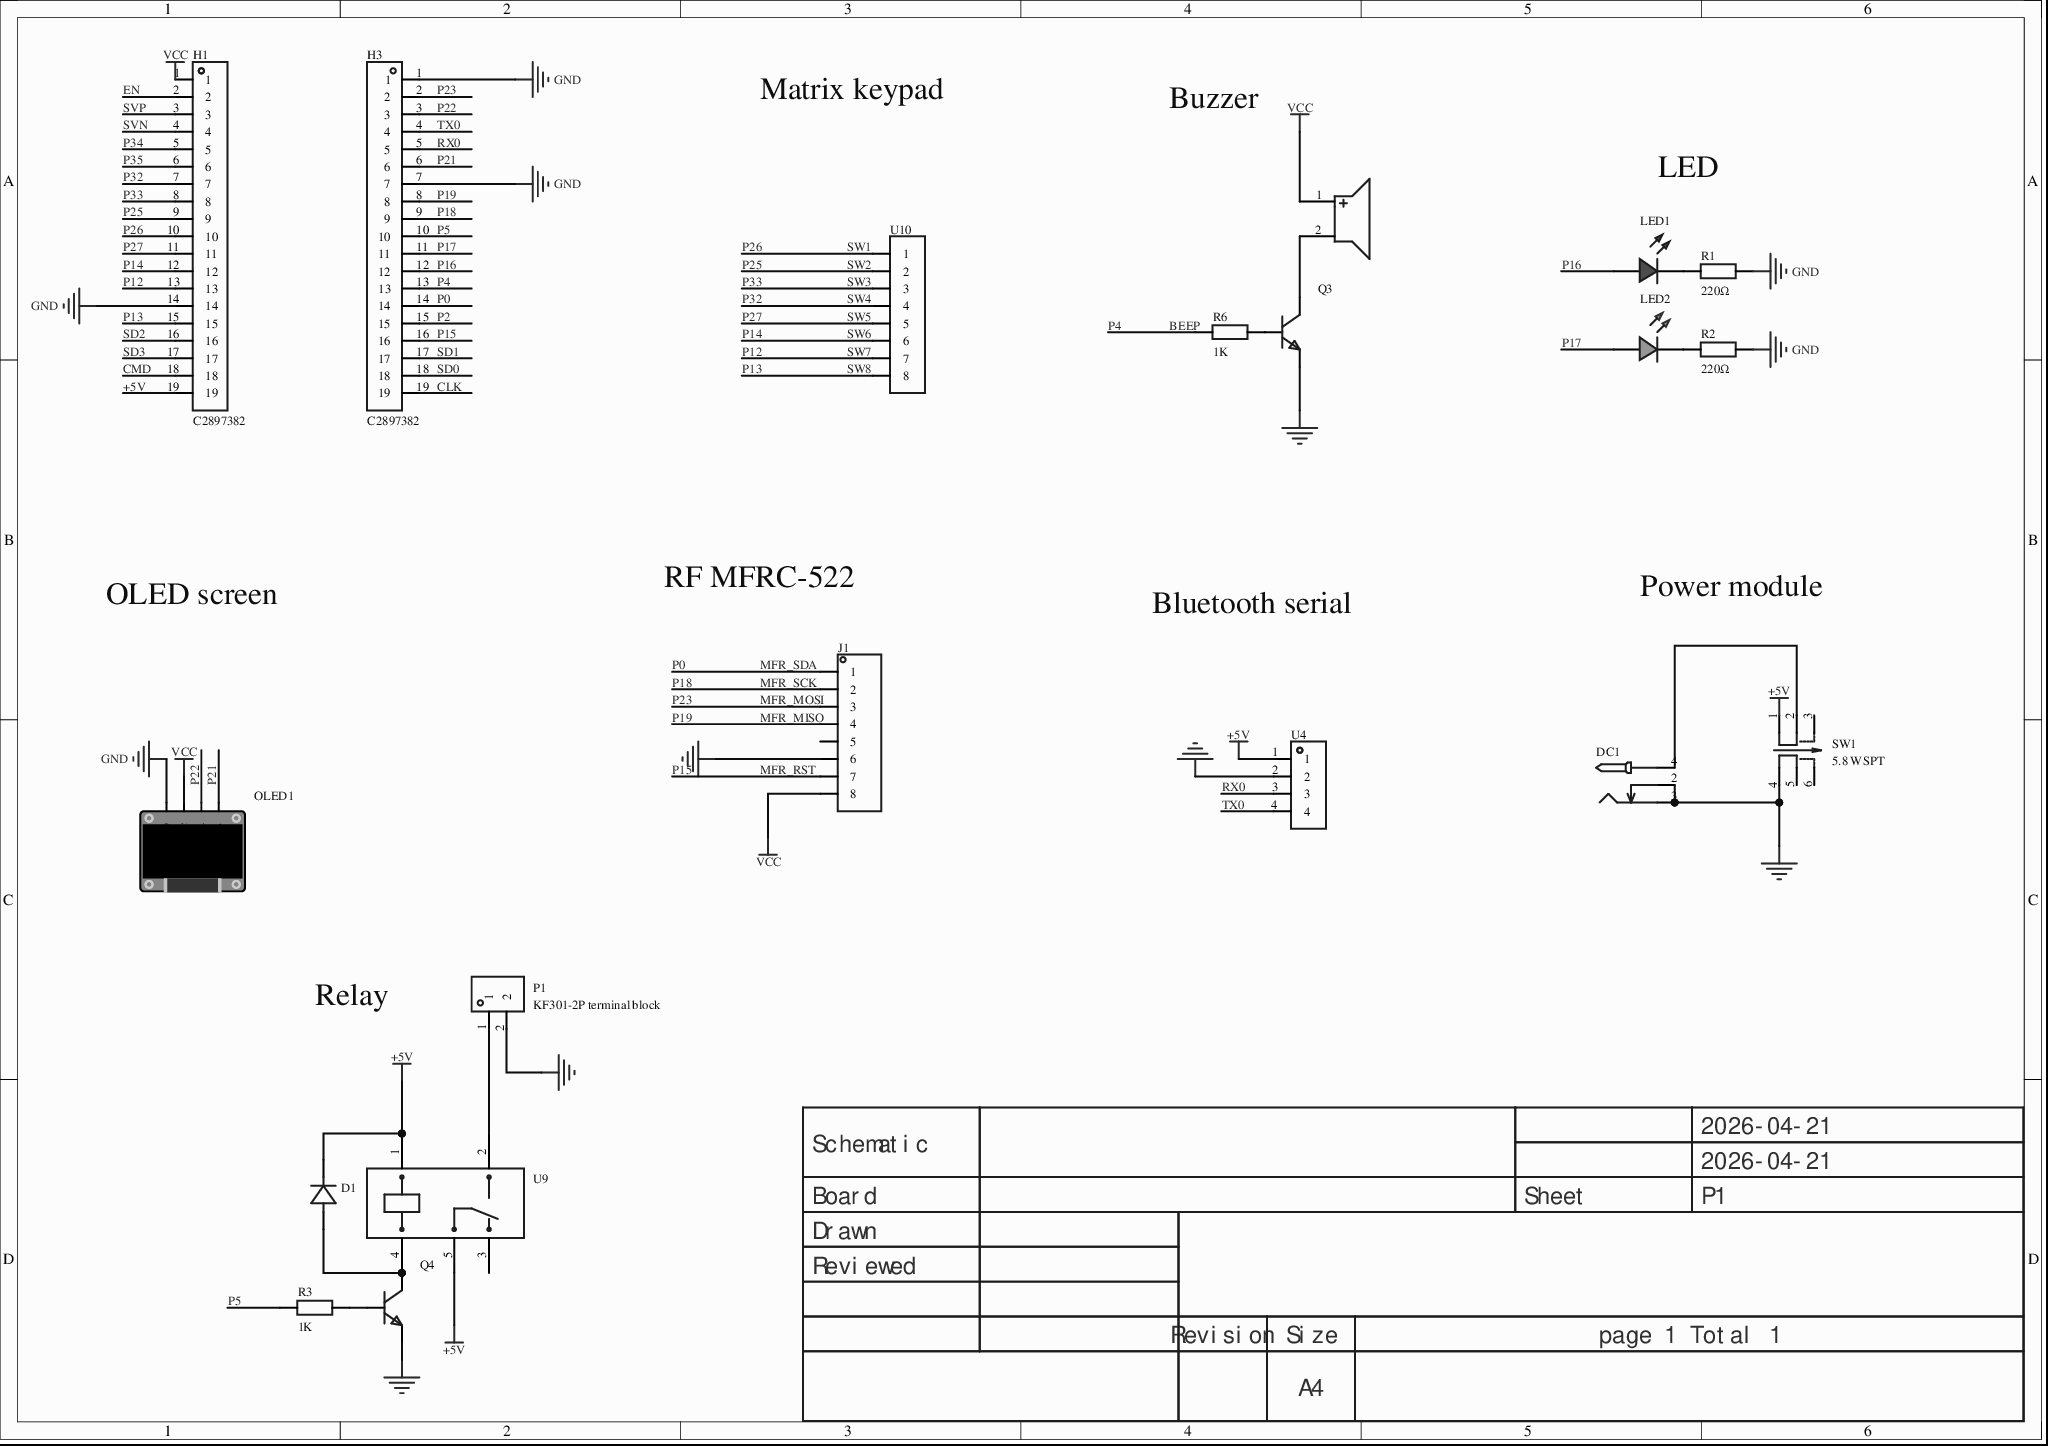
[diagram p0: MISC89084-3.schdoc]
# Altium project MISC89084-2.PrjPcb
1 sheet, 20 parts. Net scope: global (net labels, ports and power ports of the same name join across sheets).
Board file: MISC89084.pcbdoc

## Sheet MISC89084-3.schdoc
size 297 x 209 mm; Version: V1.0; @Project Name: MISC89084; @Page Count: 1; @Update Date: 2026-04-21; @Create Date: 2026-04-21; @Schematic Name: MISC89084; @Page No: 1; @Create Time: 19:02:24; @Update Time: 19:02:29; @Board Name: MISC89084

### Parts
BUZZER1  2.7kHz  [BUZ-TH_BD9.0-P4.00-D0.6-FD]  (value not drawn)
D1  (no value)  [DO_1N4007]
DC1  (no value)  [DC-2.0]
H1  C2897382  [HDR-TH_19P-P2.54-V-F]
H3  C2897382  [HDR-TH_19P-P2.54-V-F]
J1  (no value)  [HDR-TH_8P-P2.54-V-M]
LED1  (no value)  [LED_TH-3mm]
LED2  (no value)  [LED_TH-3mm]
OLED1  (no value)  [0.96OLED_4P]
P1  KF301-2P terminal block  [CONN-TH_XY301V-A-5.0-2P]
Q3  (no value)  [S8050_TO_92]
Q4  (no value)  [S8050_TO_92]
R1  220Ω  [Res_1/8W]
R2  220Ω  [Res_1/8W]
R3  1K  [Res_1/8W]
R6  1K  [Res_1/8W]
SW1  5.8 WSPT  [SW-TH_6P-L5.8-W5.8-P2.00-LS4.5-TL_K8-5851E-L1]
U4  (no value)  [HDR-TH_4P-P2.54-V-F]
U9  SRD-12VDC-SL-C  [RELAY-TH_SRD-XXVDC-XL-C]  (value not drawn)
U10  (no value)  [HDR-TH_8P-P2.54-V-F-1]

### Nets
+5V: D1.1(K) H1.19 SW1.1 U4.1 U9.1 U9.5
GND: DC1.2 DC1.3 H1.14 H3.1 H3.7 J1.6 OLED1.1(GND) P1.2 Q3.1(E) Q4.1(E) R1.2 R2.2 SW1.4 U4.2
VCC: BUZZER1.1 H1.1 J1.8 OLED1.2(VCC)
BEEP: H3.13 R6.1  [also labelled P4]
CLK: H3.19
CMD: H1.18
EN: H1.2
MFR_MISO: H3.8 J1.4  [also labelled P19]
MFR_MOSI: H3.2 J1.3  [also labelled P23]
MFR_RST: H3.16 J1.7  [also labelled P15]
MFR_SCK: H3.9 J1.2  [also labelled P18]
MFR_SDA: H3.14 J1.1  [also labelled P0]
P2: H3.15
P5: H3.10 R3.1
P12: H1.13 U10.7  [also labelled SW7]
P13: H1.15 U10.8  [also labelled SW8]
P14: H1.12 U10.6  [also labelled SW6]
P16: H3.12 LED1.1(C)
P17: H3.11 LED2.1(C)
P21: H3.6 OLED1.4(SDA)
P22: H3.3 OLED1.3(SCL)
P25: H1.9 U10.2  [also labelled SW2]
P26: H1.10 U10.1  [also labelled SW1]
P27: H1.11 U10.5  [also labelled SW5]
P32: H1.7 U10.4  [also labelled SW4]
P33: H1.8 U10.3  [also labelled SW3]
P34: H1.5
P35: H1.6
RX0: H3.5 U4.3
SD0: H3.18
SD1: H3.17
SD2: H1.16
SD3: H1.17
SVN: H1.4
SVP: H1.3
TX0: H3.4 U4.4
NetBUZZER1_2: BUZZER1.2 Q3.3(C)
NetD1_2: D1.2(A) Q4.3(C) U9.4
NetDC1_4: DC1.4 SW1.2
NetLED1_2: LED1.2(A) R1.1
NetLED2_2: LED2.2(A) R2.1
NetP1_1: P1.1 U9.2
NetQ3_2: Q3.2(B) R6.2
NetQ4_2: Q4.2(B) R3.2

Not connected (* = marked no-connect by the designer): J1 5; SW1 3 5 6; U9 3

### Notes on the sheet
- Matrix keypad
- Buzzer
- LED
- OLED screen
- RF MFRC-522
- Power module
- Bluetooth serial
- Relay
- 2026-04-21
- Schematic
- Board
- Sheet
- P1
- Drawn
- Reviewed
- Revision
- Size
- A4
- page 1 Total 1

### Library data of the parts
BUZZER1 = QMB-09B-03: Drive mode: passive (external drive); type: electromagnetic; frequency: 2.7kHz; SPL: 85dB;; Manufacturer: 华能; AddInBom: yes; ModelId: 949096c5110a440bbcfd89e7e6948986; ModelName: BUZ-TH_D9.0-H5.5-P4.0; ModelTransform: 354.33,354.33,0,90,0,0,0,0,-177.165; Voltage - Supply: 2V~5V; Symbol: QMB-09B-03; Device: QMB-09B-03; LCSC Part Name: 无源蜂鸣器QMB-09B-03; SupplierPart: C96256; ManufacturerPart: QMB-09B-03; Supplier Footprint: 插件,D=9mm; JLCPCB Part Class: Extended library; Datasheet: https://atta.szlcsc.com/upload/public/pdf/source/20210401/C96256_958B17753B5AD7CBFBCFFC7C095B4484.pdf; Supplier: LCSC; ConvertToPcb: yes; FootprintName: BUZ-TH_BD9.0-P4.00-D0.6-FD; Driver Circuitry: Passive (external drive); Technology: Electromagnetic; Value: 2.7kHz; Sound Pressure Level(SPL): 85dB; Diameter(φD): 9mm; Height: 5.7mm
D1 = D_1N4007A: AddInBom: yes; ModelId: 6de1e9b71a0d4751b4e9df530304c1a3; ModelName: DO-41_D2.4-L4.7-P8.70; ModelTransform: 373.9,94.4,232.29,0,0,0,0,0,-140; Symbol: D_1N4007; Device: D_1N4007A; Supplier Footprint: DO-41; ConvertToPcb: yes; FootprintName: DO_1N4007
DC1 = DC-005_2.0: Symbol: DC power jack; ConvertToPcb: yes; ModelId: f5f20b8a2308479b936ba3c2698865bb0819f05c4eef4c71ace90d822a990e87; ModelName: DC-IN-TH_DC-5520-1; ModelTransform: 372.05,551.18,582.68,90,0,0,137.8,0,-149.61; Device: DC-005_2.0; AddInBom: yes; Supplier Footprint: 插件; FootprintName: DC-2.0
H1 H3 = HDR-F_2.54_1x19P: ConvertToPcb: yes; ModelId: 131ee080550a465daf9368d356f53fe90819f05c4eef4c71ace90d822a990e87; ModelName: HDR-TH_19P-P2.54-F-LI-1X19P; ModelTransform: 1919.68128,95.6691,0,0,0,0,0,0,-125.984; Symbol: HDR-F_2.54_1x19P; Device: HDR-F_2.54_1x19P; AddInBom: yes; Supplier Footprint: 插件; ManufacturerPart: C2897382; FootprintName: HDR-TH_19P-P2.54-V-F
J1 = HDR-M_2.54_1x8P: Symbol: Header-Male-2.54_1x8; ConvertToPcb: yes; ModelId: f5b96e27511e49e38545e53df2320202; ModelTransform: 807.87244,98.425,0,0,0,0,0,0,-118.11; Device: HDR-M_2.54_1x8P; AddInBom: yes; SupplierPart: C124381; Supplier Footprint: 插件; FootprintName: HDR-TH_8P-P2.54-V-M; ModelName: HDR-TH_8P-P2.54-V-M
LED1 = LED_TH-R_3mm: ConvertToPcb: yes; ModelId: a497c992633541038a38947cdc58012f0819f05c4eef4c71ace90d822a990e87; ModelName: LED-TH-3mm_R; ModelTransform: 141.274,153.327,0,0,0,0,-5.984,0,-137.795; Symbol: LED_TH-R; Device: LED_TH-R_3mm; AddInBom: yes; FootprintName: LED_TH-3mm; Supplier Footprint: 插件
LED2 = LED_TH-G_3mm: AddInBom: yes; ModelId: 07c881668c9448ef9b36eb6a2126ca130819f05c4eef4c71ace90d822a990e87; ModelName: LED-TH-3mm_G; ModelTransform: 141.27444,153.32669525336098,354.32999763315956,0,0,0,-5.90551,0,-137.79528; Symbol: LED_TH-G; Device: LED_TH-G_3mm; ConvertToPcb: yes; FootprintName: LED_TH-3mm; Supplier Footprint: 插件
OLED1 = 0.96OLED模块_4P: Symbol: 0.96OLED module_4P; ConvertToPcb: yes; ModelId: 79c000fdb68d45a296c2e9bedf4f90550819f05c4eef4c71ace90d822a990e87; ModelTransform: 1393.69792,1318.895,0,0,0,0,0,-560.079,-137.795; Device: 0.96OLED module_4P; AddInBom: yes; FootprintName: 0.96OLED_4P; Supplier Footprint: 插件; ModelName: 0.96OLED_4P
P1 = KF301-2P接线端子: AddInBom: yes; ModelId: ef7ead88b0f2448d904975b26718870f0819f05c4eef4c71ace90d822a990e87; ModelTransform: 417.322,299.212,0,0,0,0,11.811,-7.835,-157.48; Symbol: KF301-2P terminal block; Device: KF301-2P terminal block; LCSC Part Name: KF301-2P接线端子; SupplierPart: C9900016950; ManufacturerPart: KF301-2P接线端子; Supplier Footprint: CK301-2P; JLCPCB Part Class: Extended Part; Supplier: LCSC; ConvertToPcb: yes; FootprintName: CONN-TH_XY301V-A-5.0-2P; ModelName: CONN-TH_XY301V-A-5.0-2P
Q3 Q4 = S8050_TO_NPN: ConvertToPcb: yes; ModelId: aafe8e06f2154e7c93506efd0d6632dd; ModelName: TO-92-3_L4.9-W3.7-P1.27-L; ModelTransform: 180.78,141.44,417.3,0,0,0,0,0,-200; Device: S8050_TO_NPN; Symbol: S8050_TO_NPN; AddInBom: yes; Supplier Footprint: TO-92; FootprintName: S8050_TO_92
R1 R2 = Res_AXIAL-1/8W: Symbol: Resistor; 3D Model: b2b5ae7ae4c642178fe0039925c86a3f; 3D Model Transform: 282.86,66.88,253.09,0,0,0,0,0,-191; ConvertToPcb: yes; ModelName: RES-TH_BD1.8-L3.2-P7.20-D0.4; Device: Res_AXIAL-1/8W; Supplier Footprint: 轴向引线; Value: 220Ω; AddInBom: yes; FootprintName: Res_1/8W
R3 = Res_AXIAL-1/8W: Symbol: Resistor; ConvertToPcb: yes; Value: 10kΩ; ModelId: b2b5ae7ae4c642178fe0039925c86a3f; ModelName: RES-TH_BD1.8-L3.2-P7.20-D0.4; ModelTransform: 282.86,66.88,253.09,0,0,0,0,0,-191; Device: Res_AXIAL-1/8W; AddInBom: yes; Supplier Footprint: 轴向引线; FootprintName: Res_1/8W
R6 = Res_AXIAL-1/8W: Symbol: Resistor; ConvertToPcb: yes; ModelId: b2b5ae7ae4c642178fe0039925c86a3f; ModelName: RES-TH_BD1.8-L3.2-P7.20-D0.4; ModelTransform: 282.86,66.88,253.09,0,0,0,0,0,-191; Value: 1K; Device: Res_AXIAL-1/8W; AddInBom: yes; Supplier Footprint: 轴向引线; FootprintName: Res_1/8W
SW1 = 5.8 WSPT: Circuit: DPDT; self-lock/no-lock: no-lock; mounting: through-hole; contact current: 100mA; rated voltage (AC): -; rated voltage (DC): 30V; with lamp: no; actuating force: 1.8N; mechanical life: 5 thousand cycles;; Manufacturer: SHOU HAN(首韩); AddInBom: yes; ModelId: b8faad98a5c645e9866333cdaba903c3; ModelTransform: 229.1334,228.346,0,0,0,0,0,0,-137.795; Actuator Style: Rectangular plunger; Insulation Resistance: 100MΩ; Actuator/Cap Color: Blue; Pin Style: PC pin; Symbol: 5.8 WSPT; Device: 5.8 WSPT; LCSC Part Name: 按键开关5.8x5.8 无锁平头 180gf; SupplierPart: C5379898; ManufacturerPart: 5.8 WSPT; Supplier Footprint: 插件; JLCPCB Part Class: Extended library; Datasheet: https://atta.szlcsc.com/upload/public/pdf/source/20230323/C831DDA43A625CDC196CB35781CDAE7F.pdf; Supplier: LCSC; ConvertToPcb: yes; FootprintName: SW-TH_6P-L5.8-W5.8-P2.00-LS4.5-TL_K8-5851E-L1; ModelName: SW-TH_6P-L5.8-W5.8-P2.00-LS4.5-TL_K8-5851E-L1; Self Lock / No Lock: No-lock; IP Rating: -; Mounting Style: Through-hole; Contact Current: 100mA; Voltage Rating (AC): -; Voltage Rating (DC): 30V; With Lamp: No; Operating Force: 1.8N; Operating Temperature: -10℃~+70℃; Mechanical Life: 5 thousand cycles
U4 = HDR-F_2.54_1x4P: Symbol: 2.54-1*4P female; ConvertToPcb: yes; ModelId: d187812051054f85879fcaa51a310d8e; ModelTransform: 419.6842,98.464,0,0,0,0,0,0,-118.11; Device: HDR-F_2.54_1x4P; AddInBom: yes; SupplierPart: C2718488; Supplier Footprint: 插件; FootprintName: HDR-TH_4P-P2.54-V-F; ModelName: HDR-TH_4P-P2.54-V-F
U9 = SRD-12VDC-SL-C: Coil voltage: 12V; contact form: 1C (SPDT changeover); contact rating (resistive): -; max switching voltage: 250V@AC; max switching current: 15A;; Manufacturer: 松乐; AddInBom: yes; ModelId: d0eda9b8bf8746d18ae810ab88dc78e7; ModelName: RELAY-TH_L19.2-W15.6-H15.8; ModelTransform: 755.904,622.4397,0,0,0,0,34.882,0,-118.11; Pin Number: 5; Coil Rated Power: 360mW; Coil Type: Non-polar, single coil; Coil Resistance: 400Ω; Contact Resistance: 100mΩ; Operate Time: 10ms; Symbol: SRD-12VDC-SL-C; Device: SRD-12VDC-SL-C; LCSC Part Name: SRD-12VDC-SL-C; SupplierPart: C30431; ManufacturerPart: SRD-12VDC-SL-C; Supplier Footprint: 插件,15.6x19.2mm; JLCPCB Part Class: Extended library; Datasheet: https://atta.szlcsc.com/upload/public/pdf/source/20200305/C490149_C96E4098A3B1FFB377D5AD2E40B7C2A8.pdf; Supplier: LCSC; ConvertToPcb: yes; FootprintName: RELAY-TH_SRD-XXVDC-XL-C; Coil Voltage: 12V; Contact Form: 1C (SPDT changeover); Contact Rating: -; Maximum Switching Voltage: 250V@AC; Maximum Switching Current: 15A; Release Time: 10ms
U10 = HDR-F_2.54_1x8P: Symbol: Header-Female-2.54_1x8; AddInBom: yes; ModelId: 0f7e4d9227ef4fa08d5469c22cc70cdb; ModelName: HDR-F-2.54_1x8; ModelTransform: 799.99844,100,0,0,0,0,0,0,-118.11; Device: HDR-F_2.54_1x8P; ConvertToPcb: yes; FootprintName: HDR-TH_8P-P2.54-V-F-1; SupplierPart: C27438; Supplier Footprint: 插件